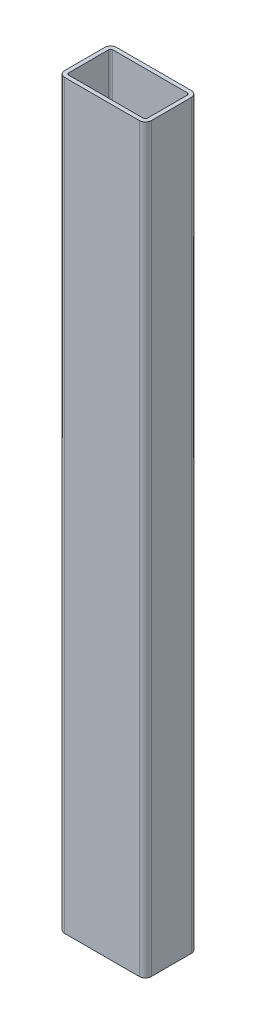
SolidWorks part; units mm, degrees
ref_plane "Front" through (0, 0, 0) normal (0, 0, 1) x (1, 0, 0)
ref_plane "Top" through (0, 0, 0) normal (0, 1, 0) x (1, 0, 0)
ref_plane "Right" through (0, 0, 0) normal (1, 0, 0) x (0, 0, -1)
sketch "Sketch1" plane through (0, 0, 0) normal (0, 1, 0) x (1, 0, 0)
  line L0 (-21.55, -12.7) -> (21.55, -12.7)
  line L1 (-21.55, -15) -> (21.55, -15)
  line L2 (-25, -11.55) -> (-25, 11.55)
  line L3 (-21.55, 15) -> (21.55, 15)
  line L4 (25, -11.55) -> (25, 11.55)
  line L5 (-25, -15) -> (25, 15) construction
  line L6 (-25, 15) -> (25, -15) construction
  line L7 (22.7, -11.55) -> (22.7, 11.55)
  line L8 (-21.55, 12.7) -> (21.55, 12.7)
  line L9 (-22.7, -11.55) -> (-22.7, 11.55)
  arc A0 (21.55, 15) -> (25, 11.55) centre (21.55, 11.55) cw
  arc A1 (-21.55, -15) -> (-25, -11.55) centre (-21.55, -11.55) cw
  arc A2 (21.55, -15) -> (25, -11.55) centre (21.55, -11.55) ccw
  arc A3 (-25, 11.55) -> (-21.55, 15) centre (-21.55, 11.55) cw
  arc A4 (21.55, -12.7) -> (22.7, -11.55) centre (21.55, -11.55) ccw
  arc A5 (21.55, 12.7) -> (22.7, 11.55) centre (21.55, 11.55) cw
  arc A6 (-22.7, 11.55) -> (-21.55, 12.7) centre (-21.55, 11.55) cw
  arc A7 (-21.55, -12.7) -> (-22.7, -11.55) centre (-21.55, -11.55) cw
  point P0 (0, 0)
  dimension "D3" = 3.45
  dimension "D1" = 50
  dimension "D2" = 30
  dimension "D4" = 2.3
extrude "Boss-Extrude1" add sketch "Sketch1" along normal blind 428
